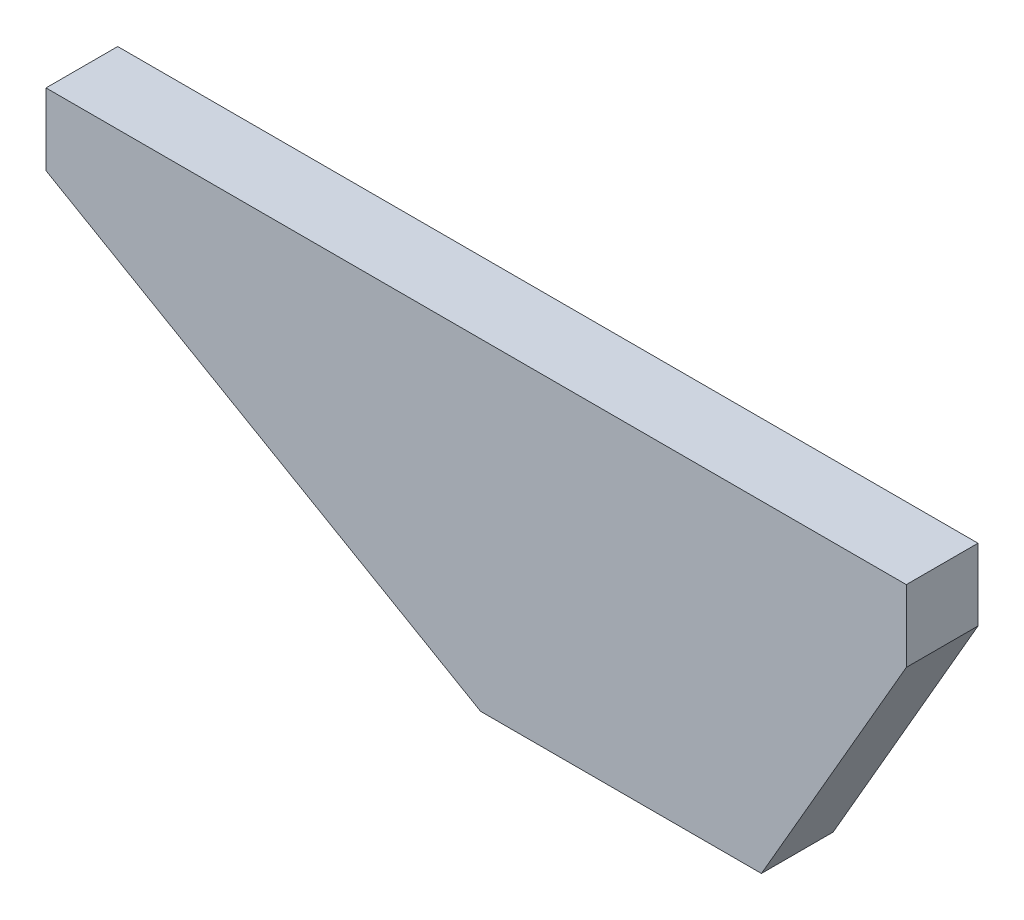
from build123d import *

# Parameters (mm, degrees)
BOSS_EXTRUDE1_DEPTH = 10


with BuildPart() as part:
    # Sketch1 → Boss-Extrude1 (new body)
    with BuildSketch(Plane.XY):
        Polygon((0, 0), (120, 0), (120, -10), (99.792740578, -45), (60.621778265, -45), (0, -10), align=None)
    extrude(amount=BOSS_EXTRUDE1_DEPTH)


solid = part.part
